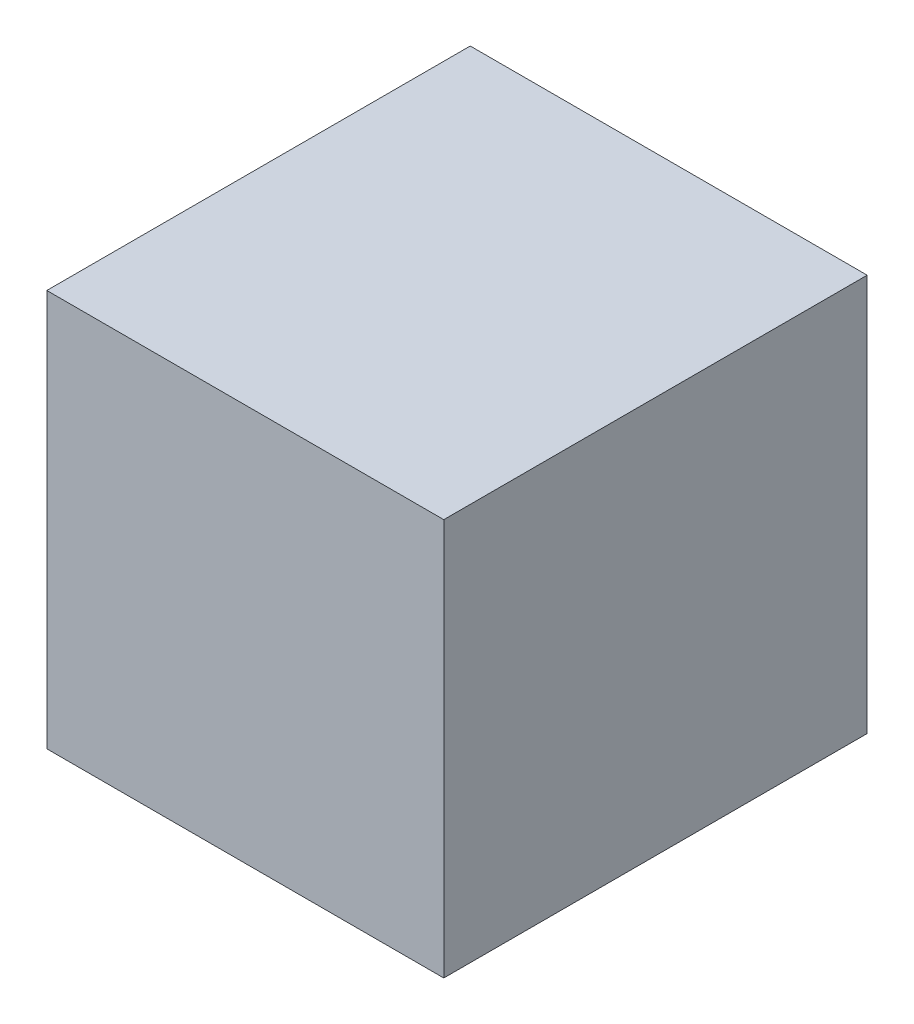
from build123d import *

# Parameters (mm, degrees)
SKETCH_1_W             = 75
SKETCH_1_H             = 75
EXTRUDE_1_DEPTH        = 80
HOLE_WIZARD_M6_2_D     = 5
HOLE_WIZARD_M6_2_DEPTH = 15
HOLE_WIZARD_M6_2_TIP   = 1.502151548


with BuildPart() as part:
    # 草图1 → 凸台-拉伸1 (new body)
    with BuildSketch(Plane.XY):
        Rectangle(SKETCH_1_W, SKETCH_1_H)
    extrude(amount=EXTRUDE_1_DEPTH)

    # M6 螺纹孔2
    with Locations(Plane(origin=(0, 0, 0), x_dir=(-1, 0, 0), z_dir=(0, 0, -1))):
        with Locations((-31.5, 31), (-20.5, 31), (20.5, 31), (20.5, -31), (-20.5, -31), (-31.5, -31)):
            Hole(HOLE_WIZARD_M6_2_D / 2, depth=HOLE_WIZARD_M6_2_DEPTH)
            with Locations((0, 0, -(HOLE_WIZARD_M6_2_DEPTH + HOLE_WIZARD_M6_2_TIP / 2))):  # 118° drill point
                Cone(0, HOLE_WIZARD_M6_2_D / 2, HOLE_WIZARD_M6_2_TIP, mode=Mode.SUBTRACT)


solid = part.part
